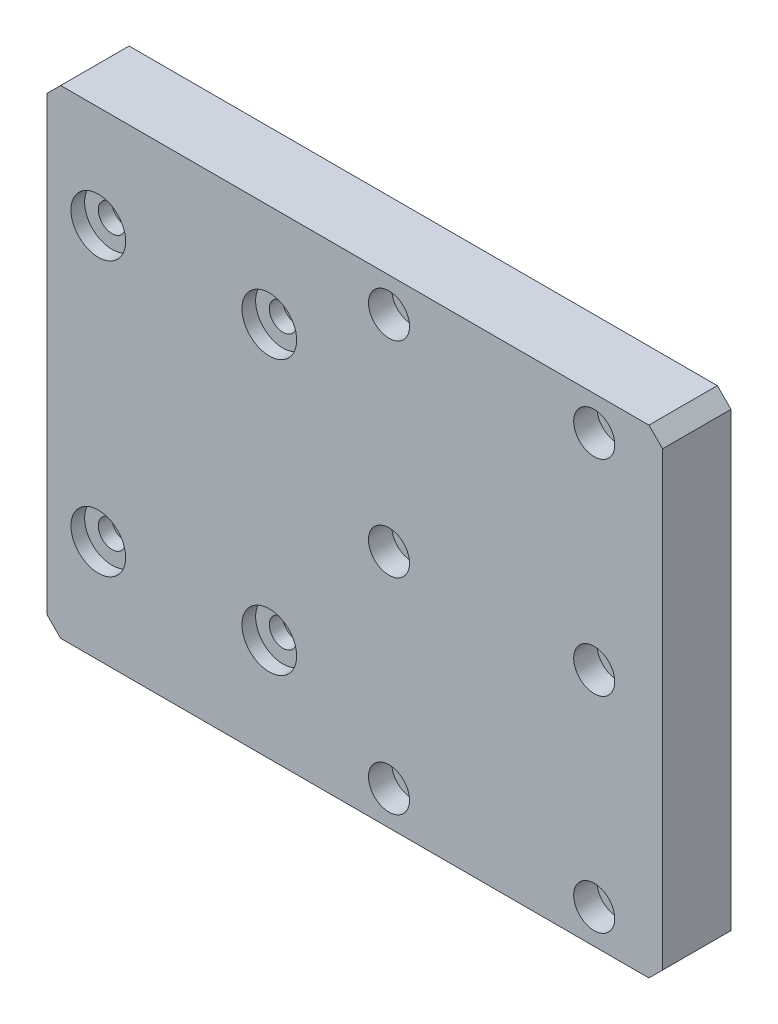
SolidWorks part; units mm, degrees
material "6061-T6 (SS)"
ref_plane "前基準面" through (0, 0, 0) normal (0, 0, 1) x (1, 0, 0)
ref_plane "上基準面" through (0, 0, 0) normal (0, 1, 0) x (1, 0, 0)
ref_plane "右基準面" through (0, 0, 0) normal (1, 0, 0) x (0, 0, -1)
sketch "草图1" plane through (0, 0, 0) normal (0, 0, 1) x (1, 0, 0)
  line L1 (-45, -35) -> (45, -35)
  line L2 (-45, -35) -> (-45, 35)
  line L3 (-45, 35) -> (45, 35)
  line L4 (45, -35) -> (45, 35)
  line L5 (-45, -35) -> (45, 35) construction
  line L6 (-45, 35) -> (45, -35) construction
  point P0 (0, 0)
  dimension "D1" = 90
  dimension "D2" = 70
extrude "凸台-拉伸1" add sketch "草图1" along normal mid plane 10
hole_wizard "打孔尺寸(%根据)内六角圆柱头螺钉的类型1" positions "草图2" profile "草图3" counterbore size "M3" standard "GB" end condition through all
sketch "草图2" plane through (0, 0, 5) normal (0, 0, 1) x (1, 0, 0)
  line L0 (0, 0) -> (-57.1626, 0) construction
  line L4 (45, -35) -> (45, 35) construction
  point P0 (5, 30)
  point P2 (5, 0)
  point P4 (5, -30)
  point P17 (35, 30)
  point P19 (35, 0)
  point P21 (35, -30)
  dimension "D1" = 30
  dimension "D2" = 30
  dimension "D3" = 10
sketch "草图3" plane through (5, 30, 5) normal (1, 0, 0) x (0, -1, 0)
  line L0 (0, 0) -> (0, 10)
  line L1 (0, 10) -> (1.7, 10)
  line L3 (1.7, 10) -> (1.7, 3.4)
  line L4 (1.7, 3.4) -> (3, 3.4)
  line L5 (3, 3.4) -> (3, 0)
  line L7 (3, 0) -> (0, 0)
  line L11 (0, -6.35) -> (0, 107.95) construction
  dimension "通孔孔直径" = 3.4
  dimension "通孔孔深度" = 10
  dimension "柱形沉头孔直径" = 6
  dimension "柱形沉头孔深度" = 3.4
hole_wizard "打孔尺寸(%根据)内六角圆柱头螺钉的类型3" positions "草图4" profile "草图5" counterbore size "M3" standard "GB" end condition through all
sketch "草图4" plane through (0, 0, -5) normal (0, 0, -1) x (-1, 0, 0)
  line L0 (0, 0) -> (59.2041, 0) construction
  line L3 (0, 0) -> (0, 43.3333) construction
  line L6 (45, 35) -> (45, -35) construction
  point P0 (37.5, 20)
  point P2 (12.5, 20)
  point P4 (12.5, -20)
  point P6 (37.5, -20)
  dimension "D1" = 25
  dimension "D2" = 40
  dimension "D3" = 7.5
sketch "草图5" plane through (-37.5, 20, -5) normal (1, 0, 0) x (0, 1, 0)
  line L0 (0, 0) -> (0, 10)
  line L1 (0, 10) -> (1.6, 10)
  line L3 (1.6, 10) -> (1.6, 3.4)
  line L4 (1.6, 3.4) -> (3, 3.4)
  line L5 (3, 3.4) -> (3, 0)
  line L7 (3, 0) -> (0, 0)
  line L11 (0, -6.35) -> (0, 107.95) construction
  dimension "通孔孔直径" = 3.2
  dimension "通孔孔深度" = 10
  dimension "柱形沉头孔直径" = 6
  dimension "柱形沉头孔深度" = 3.4
sketch "草图6" plane through (0, 0, 5) normal (0, 0, 1) x (1, 0, 0)
  circle A0 centre (-37.5, 20) radius 4
  circle A1 centre (-12.5, 20) radius 4
  circle A2 centre (-37.5, -20) radius 4
  circle A3 centre (-12.5, -20) radius 4
  dimension "D1" = 8
extrude "切除-拉伸1" cut sketch "草图6" against normal blind 2
sketch "草图8" plane through (0, 0, 3) normal (0, 0, 1) x (1, 0, 0)
  circle A0 centre (-37.5, 20) radius 2
  circle A1 centre (-37.5, -20) radius 2
  circle A2 centre (-12.5, -20) radius 2
  circle A3 centre (-12.5, 20) radius 2
  dimension "D1" = 4
extrude "切除-拉伸2" cut sketch "草图8" against normal blind 2
chamfer "倒角1" distance 2 angle 45 4 edges at (-45, -35, 0) (45, -35, 0) (45, 35, 0) (-45, 35, 0)
